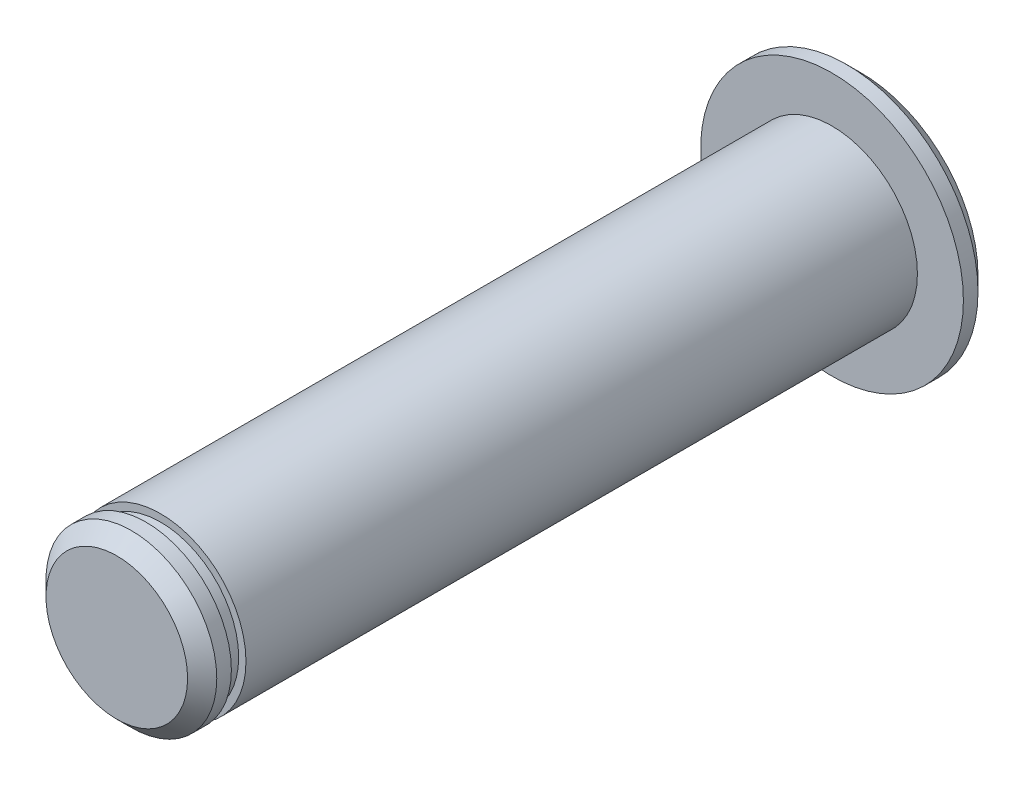
SolidWorks part; units mm, degrees
ref_plane "Front Plane" through (0, 0, 0) normal (0, 0, 1) x (1, 0, 0)
ref_plane "Top Plane" through (0, 0, 0) normal (0, 1, 0) x (1, 0, 0)
ref_plane "Right Plane" through (0, 0, 0) normal (1, 0, 0) x (0, 0, -1)
sketch "Sketch1" plane through (0, 0, 0) normal (0, 0, 1) x (1, 0, 0)
  circle A0 centre (0, 0) radius 9
  dimension "D1" = 18
extrude "Boss-Extrude1" add sketch "Sketch1" along normal blind 2
sketch "Sketch2" plane through (0, 0, 2) normal (0, 0, 1) x (1, 0, 0)
  circle A0 centre (0, 0) radius 5.85
  dimension "D1" = 11.7
extrude "Boss-Extrude2" add sketch "Sketch2" along normal blind 46
sketch "Sketch4" plane through (0, 0, 48) normal (0, 0, 1) x (1, 0, 0)
  circle A0 centre (0, 0) radius 5.35
  dimension "D1" = 10.7
extrude "Boss-Extrude3" add sketch "Sketch4" along normal blind 1
sketch "Sketch5" plane through (0, 0, 49) normal (0, 0, 1) x (1, 0, 0)
  circle A0 centre (0, 0) radius 5.85
  dimension "D1" = 11.7
extrude "Boss-Extrude4" add sketch "Sketch5" along normal blind 2
chamfer "Chamfer1" distance 1 angle 45 2 edges at (9, 0, 0) (5.85, 0, 51)
